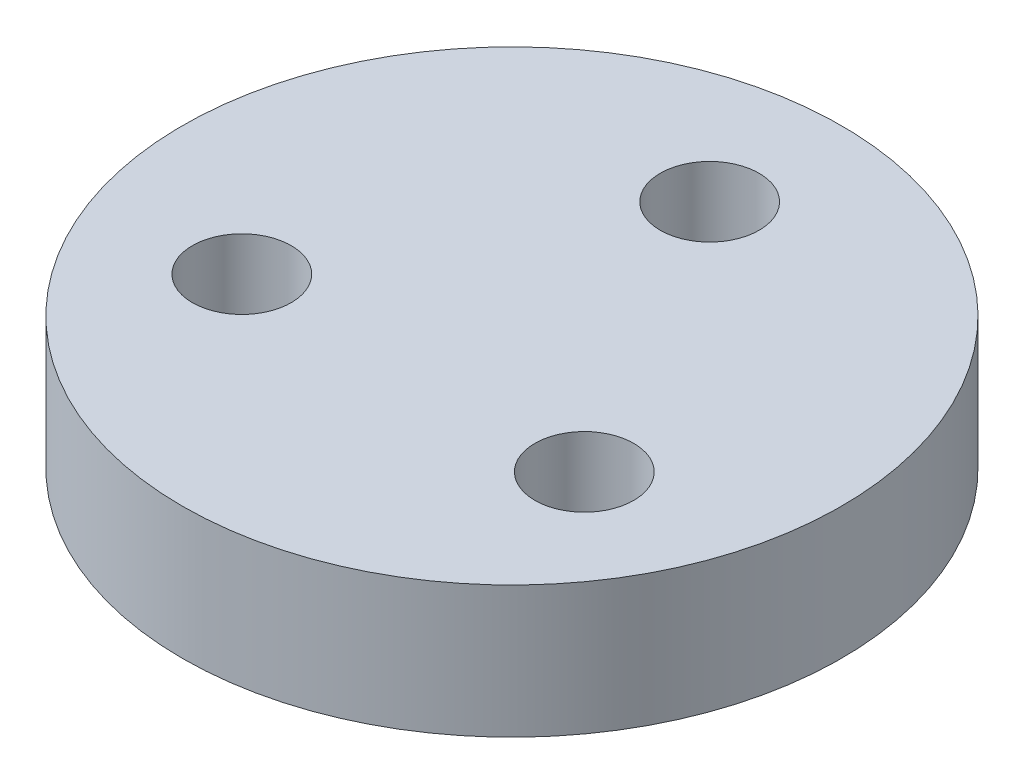
from build123d import *

# Parameters (mm, degrees)
SKETCH1_R           = 50
BOSS_EXTRUDE1_DEPTH = 20
SKETCH2_R           = 7.5
CUT_EXTRUDE1_DEPTH  = 15
SKETCH3_R           = 1
CUT_EXTRUDE2_DEPTH  = 74.484692283
SKETCH4_R           = 1.8
CUT_EXTRUDE3_DEPTH  = 4


with BuildPart() as part:
    # Sketch1 → Boss-Extrude1 (new body)
    with BuildSketch(Plane(origin=(0, 0, 0), x_dir=(1, 0, 0), z_dir=(0, 1, 0))):
        with Locations(Location((0, 0, 0), (0, 0, 270))):
            Circle(SKETCH1_R)
    extrude(amount=BOSS_EXTRUDE1_DEPTH)

    # Sketch2 → Cut-Extrude1 (cut)
    with BuildSketch(Plane(origin=(0, 20, 0), x_dir=(1, 0, 0), z_dir=(0, 1, 0))):
        with Locations(Location((0, 30, 0), (0, 0, 270))):
            Circle(SKETCH2_R)
        with Locations(Location((25.980762114, -15, 0), (0, 0, 270))):
            Circle(SKETCH2_R)
        with Locations(Location((-25.980762114, -15, 0), (0, 0, 270))):
            Circle(SKETCH2_R)
    extrude(amount=-CUT_EXTRUDE1_DEPTH, mode=Mode.SUBTRACT)

    # Sketch3 → Cut-Extrude2 (cut, through all)
    with BuildSketch(Plane.XZ):
        with Locations(Location((25.980762114, 19, 0), (0, 0, 270))):
            Circle(SKETCH3_R)
        with Locations(Location((29.980762114, 15, 0), (0, 0, 270))):
            Circle(SKETCH3_R)
        with Locations(Location((21.980762114, 15, 0), (0, 0, 270))):
            Circle(SKETCH3_R)
        with Locations(Location((25.980762114, 11, 0), (0, 0, 270))):
            Circle(SKETCH3_R)
        with Locations(Location((-25.980762114, 19, 0), (0, 0, 270))):
            Circle(SKETCH3_R)
        with Locations(Location((-29.980762114, 15, 0), (0, 0, 270))):
            Circle(SKETCH3_R)
        with Locations(Location((-25.980762114, 11, 0), (0, 0, 270))):
            Circle(SKETCH3_R)
        with Locations(Location((-21.980762114, 15, 0), (0, 0, 270))):
            Circle(SKETCH3_R)
        with Locations(Location((0, -26, 0), (0, 0, 270))):
            Circle(SKETCH3_R)
        with Locations(Location((-4, -30, 0), (0, 0, 270))):
            Circle(SKETCH3_R)
        with Locations(Location((0, -34, 0), (0, 0, 270))):
            Circle(SKETCH3_R)
        with Locations(Location((4, -30, 0), (0, 0, 270))):
            Circle(SKETCH3_R)
    extrude(amount=-CUT_EXTRUDE2_DEPTH, mode=Mode.SUBTRACT)

    # Sketch4 → Cut-Extrude3 (cut)
    with BuildSketch(Plane.XZ):
        with Locations(Location((-25.980762114, 19, 0), (0, 0, 270))):
            Circle(SKETCH4_R)
        with Locations(Location((-29.980762114, 15, 0), (0, 0, 270))):
            Circle(SKETCH4_R)
        with Locations(Location((-25.980762114, 11, 0), (0, 0, 270))):
            Circle(SKETCH4_R)
        with Locations(Location((-21.980762114, 15, 0), (0, 0, 270))):
            Circle(SKETCH4_R)
        with Locations(Location((25.980762114, 19, 0), (0, 0, 270))):
            Circle(SKETCH4_R)
        with Locations(Location((21.980762114, 15, 0), (0, 0, 270))):
            Circle(SKETCH4_R)
        with Locations(Location((25.980762114, 11, 0), (0, 0, 270))):
            Circle(SKETCH4_R)
        with Locations(Location((29.980762114, 15, 0), (0, 0, 270))):
            Circle(SKETCH4_R)
        with Locations(Location((0, -26, 0), (0, 0, 270))):
            Circle(SKETCH4_R)
        with Locations(Location((-4, -30, 0), (0, 0, 270))):
            Circle(SKETCH4_R)
        with Locations(Location((0, -34, 0), (0, 0, 270))):
            Circle(SKETCH4_R)
        with Locations(Location((4, -30, 0), (0, 0, 270))):
            Circle(SKETCH4_R)
    extrude(amount=-CUT_EXTRUDE3_DEPTH, mode=Mode.SUBTRACT)


solid = part.part
